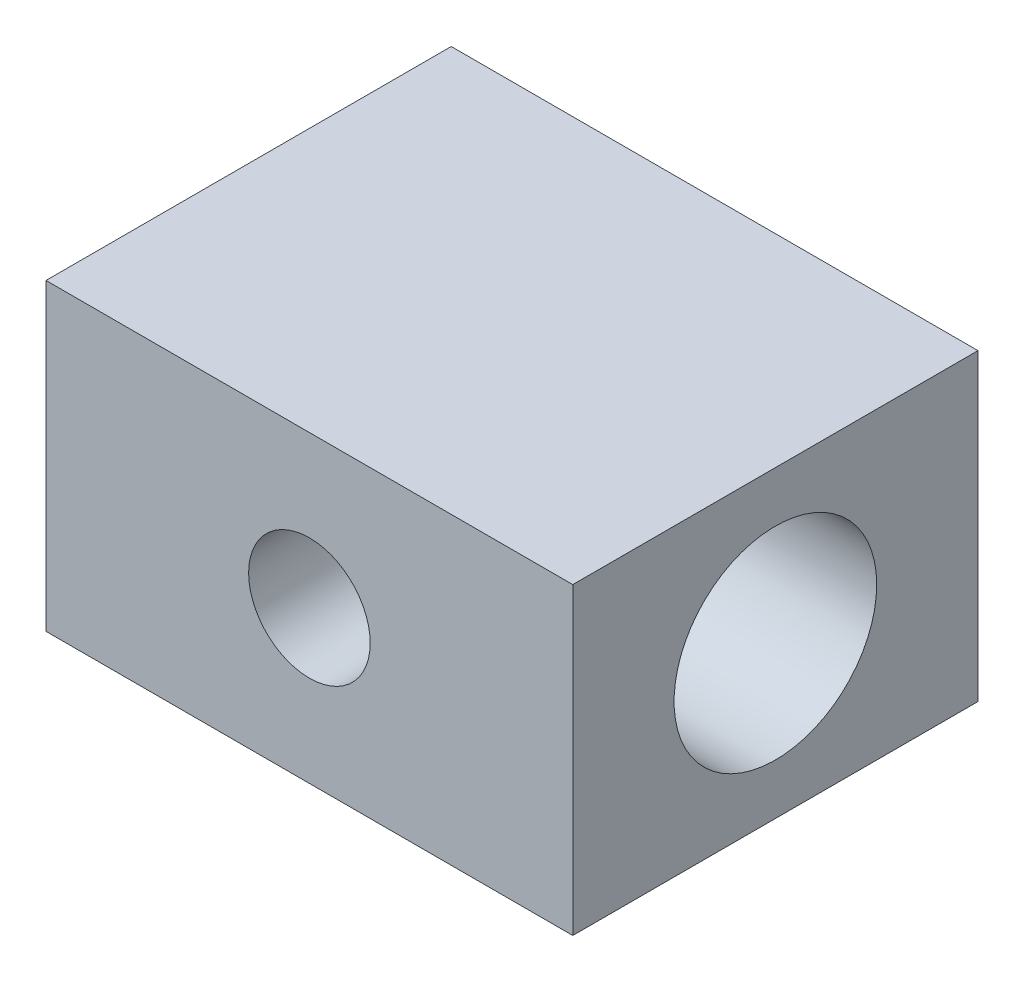
SolidWorks part; units mm, degrees
ref_plane "Front Plane" through (0, 0, 0) normal (0, 0, 1) x (1, 0, 0)
ref_plane "Top Plane" through (0, 0, 0) normal (0, 1, 0) x (1, 0, 0)
ref_plane "Right Plane" through (0, 0, 0) normal (1, 0, 0) x (0, 0, -1)
sketch "Sketch1" plane through (0, 0, 0) normal (0, 0, 1) x (1, 0, 0)
  line L1 (-13, 7.5) -> (13, 7.5)
  line L2 (-13, 7.5) -> (-13, -7.5)
  line L3 (-13, -7.5) -> (13, -7.5)
  line L4 (13, 7.5) -> (13, -7.5)
  line L5 (-13, 7.5) -> (13, -7.5) construction
  line L6 (-13, -7.5) -> (13, 7.5) construction
  circle A0 centre (0, 0) radius 3
  point P0 (0, 0)
  dimension "D3" = 6
  dimension "D1" = 26
  dimension "D2" = 15
extrude "Boss-Extrude1" add sketch "Sketch1" along normal blind 20
sketch "Sketch2" plane through (13, 0, 0) normal (1, 0, 0) x (0, 0, -1)
  circle A0 centre (-10, 0) radius 5
  dimension "D1" = 10
extrude "Cut-Extrude1" cut sketch "Sketch2" against normal through all
